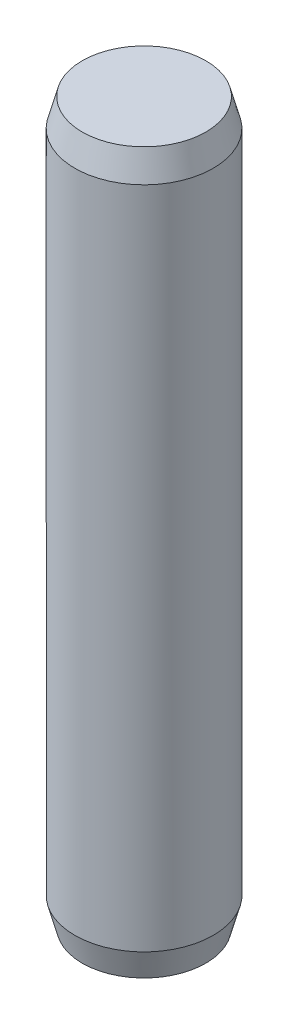
SolidWorks part; units mm, degrees
ref_plane "Front Plane" through (0, 0, 0) normal (0, 0, 1) x (1, 0, 0)
ref_plane "Top Plane" through (0, 0, 0) normal (0, 1, 0) x (1, 0, 0)
ref_plane "Right Plane" through (0, 0, 0) normal (1, 0, 0) x (0, 0, -1)
other "Configuration Table"
sketch "Sketch1" plane through (0, 0, 0) normal (0, 1, 0) x (1, 0, 0)
  circle A0 centre (0, 0) radius 2.5
  dimension "D1" = 5
extrude "Boss-Extrude1" add sketch "Sketch1" along normal mid plane 26
chamfer "Chamfer1" distance 1 angle 15 1 edges at (0, 13, 2.5)
chamfer "Chamfer3" distance 0.27 angle 75 1 edges at (0, -13, 2.5)
